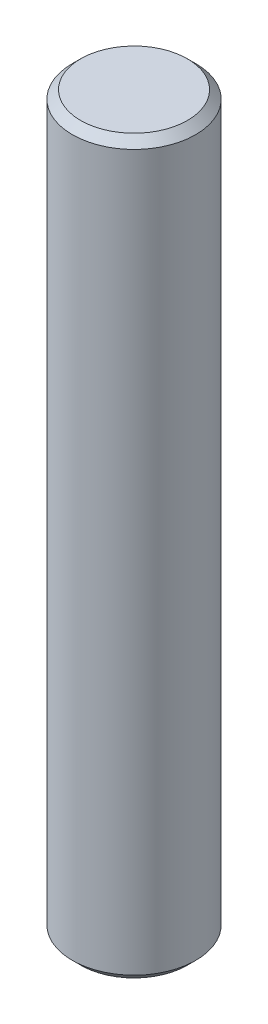
from build123d import *

# Parameters (mm, degrees)
SKETCH1_W     = 15
SKETCH1_H     = 178
CHAMFER1_SIZE = 2


with BuildPart() as part:
    # Sketch1 → Revolve1 (revolve)
    with BuildSketch(Plane.XY, mode=Mode.PRIVATE) as revolve1_sk:
        with Locations((7.5, 89)):
            Rectangle(SKETCH1_W, SKETCH1_H)
    revolve(revolve1_sk.sketch.rotate(Axis((0, 0, 0), (0, 1, 0)), 90), axis=Axis((0, 0, 0), (0, 1, 0)))

    # Chamfer1
    chamfer1_edges = [part.edges().sort_by_distance(p)[0] for p in [
        (0, 178, 15),
        (0, 0, 15),
    ]]
    chamfer(chamfer1_edges, length=CHAMFER1_SIZE)


solid = part.part
